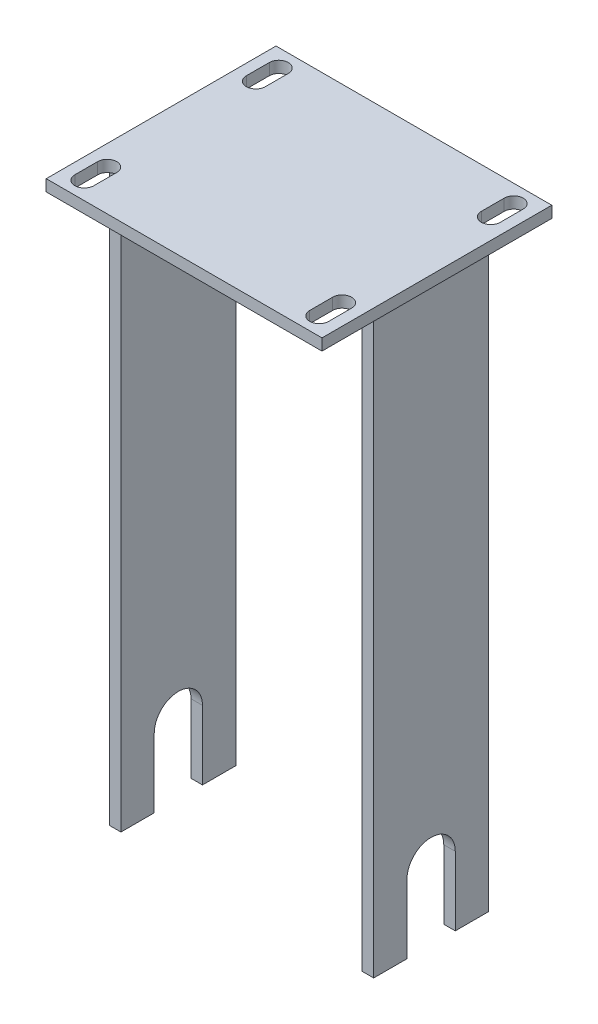
from build123d import *

# Parameters (mm, degrees)
SKETCH1_W            = 120
SKETCH1_H            = 100
BOSS_EXTRUDE1_DEPTH  = 5
CUT_EXTRUDE1_DEPTH   = 157.284996081
MIRROR2_COPY_1_DEPTH = 157.284996081
BOSS_EXTRUDE2_DEPTH  = 250
CUT_EXTRUDE2_DEPTH   = 450


with BuildPart() as part:
    # Sketch1 → Boss-Extrude1 (new body)
    with BuildSketch(Plane(origin=(0, 0, 0), x_dir=(1, 0, 0), z_dir=(0, 1, 0))):
        with Locations((60, 50)):
            Rectangle(SKETCH1_W, SKETCH1_H)
    extrude(amount=BOSS_EXTRUDE1_DEPTH)

    # Sketch2 → Cut-Extrude1 (cut, through all)
    with BuildSketch(Plane(origin=(0, 5, 0), x_dir=(1, 0, 0), z_dir=(0, 1, 0))):
        with BuildLine():
            Line((13.012661712, 92.320396367), (13.012661712, 82.342416735))
            ThreePointArc((13.012661712, 82.342416735), (8.883842554, 78.213597578), (4.755023397, 82.342416735))
            Line((4.755023397, 82.342416735), (4.755023397, 92.320396367))
            ThreePointArc((4.755023397, 92.320396367), (8.883842554, 96.449215524), (13.012661712, 92.320396367))
        make_face()
    cut_extrude1 = extrude(amount=-CUT_EXTRUDE1_DEPTH, mode=Mode.SUBTRACT)

    # Mirror1: Cut-Extrude1 across plane
    add(cut_extrude1.mirror(Plane.ZY.offset(-60)), mode=Mode.SUBTRACT)

    # Mirror2: Cut-Extrude1 across plane
    add(cut_extrude1.mirror(Plane.XY.offset(-50)), mode=Mode.SUBTRACT)

    # Mirror2 copy 1 sketch → Mirror2 copy 1 (cut, through all)
    with BuildSketch(Plane(origin=(120, 5, -100), x_dir=(-1, 0, 0), z_dir=(0, 1, 0))):
        with BuildLine():
            Line((13.012661712, 92.320396367), (13.012661712, 82.342416735))
            ThreePointArc((13.012661712, 82.342416735), (8.883842554, 78.213597578), (4.755023397, 82.342416735))
            Line((4.755023397, 82.342416735), (4.755023397, 92.320396367))
            ThreePointArc((4.755023397, 92.320396367), (8.883842554, 96.449215524), (13.012661712, 92.320396367))
        make_face()
    extrude(amount=-MIRROR2_COPY_1_DEPTH, mode=Mode.SUBTRACT)

    # Sketch4 → Boss-Extrude2 (add)
    with BuildSketch(Plane.XZ):
        Polygon((2.5, -50), (2.5, -75), (7.5, -75), (7.5, -50), (7.5, -25), (2.5, -25), align=None)
        Polygon((112.5, -75), (117.5, -75), (117.5, -45), (117.5, -25), (112.5, -25), (112.5, -45), align=None)
    extrude(amount=BOSS_EXTRUDE2_DEPTH)

    # Sketch5 → Cut-Extrude2 (cut)
    with BuildSketch(Plane.ZY.offset(-2.5)):
        with BuildLine():
            Line((-60.5, -250), (-60.5, -220))
            ThreePointArc((-60.5, -220), (-50, -209.5), (-39.5, -220))
            Line((-39.5, -220), (-39.5, -250))
            ThreePointArc((-39.5, -250), (-50, -260.5), (-60.5, -250))
        make_face()
    extrude(amount=-CUT_EXTRUDE2_DEPTH, mode=Mode.SUBTRACT)


solid = part.part
